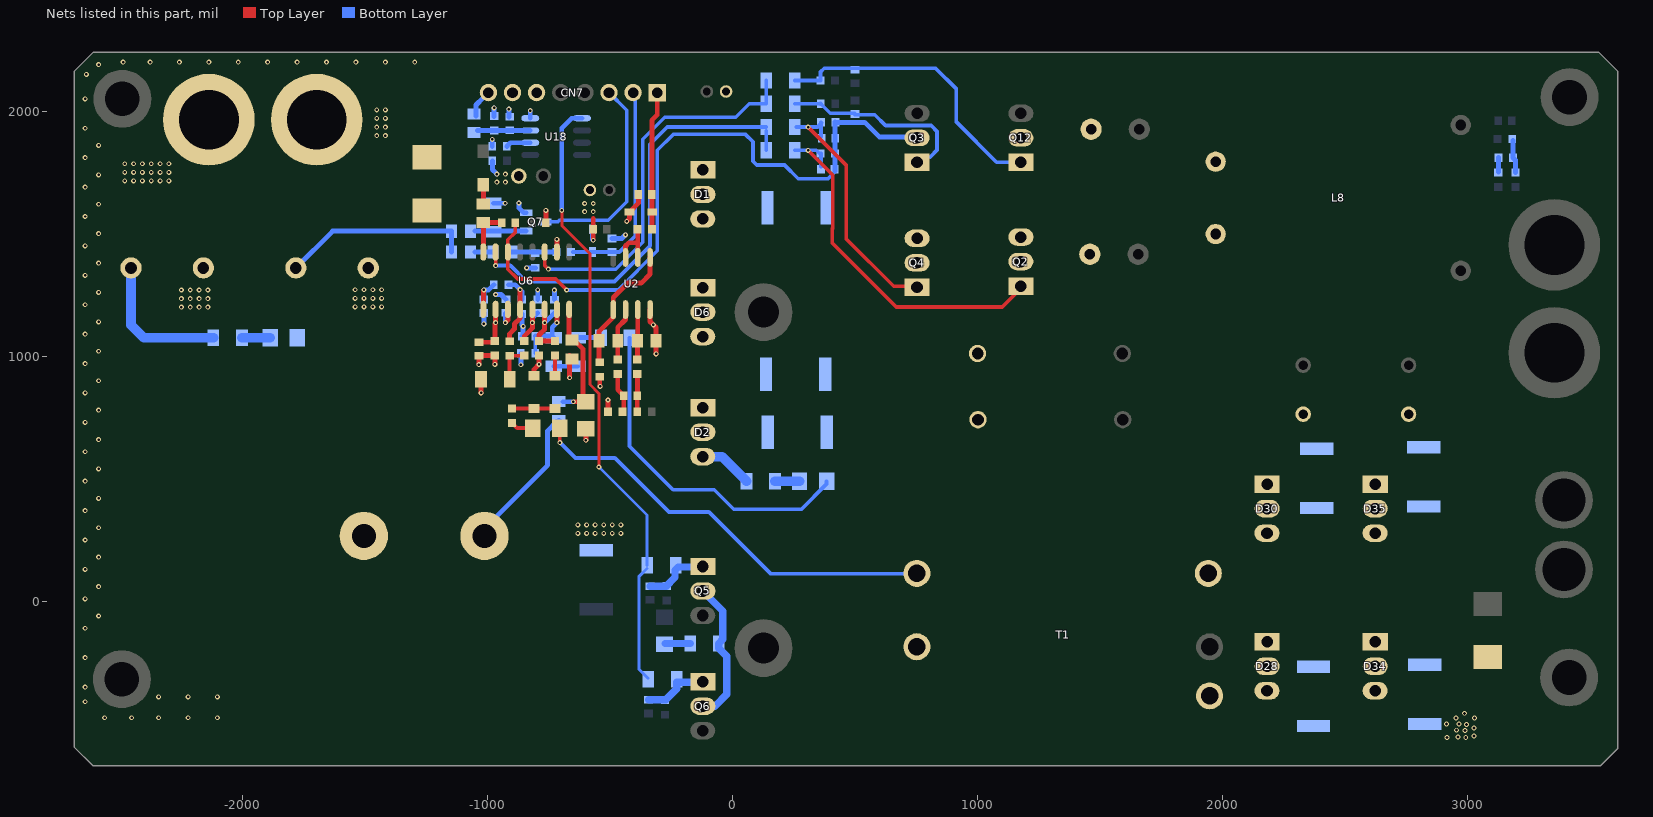
[diagram p0: the nets of this part, all layers, seen from the top]
# Altium PCB MISC89356.PcbDoc (part 2 of 3)
Units mil, origin at the board's own origin, x right, y up, seen from the top; angles counter-clockwise.
Board outline 6299.21 x 2912.91 mil, 4 copper layers (Top Layer, GND02, PWR03, Bottom Layer); 128 components, 68 nets, 313 pads, 200 vias.

## Via types
v1: diameter 20, hole 10, Top Layer to Bottom Layer, tented both sides, 177 vias
v2: diameter 20, hole 12, Top Layer to Bottom Layer, 13 vias
v3: diameter 20, hole 10, Top Layer to Bottom Layer, 10 vias

## Nets (pads, with @x,y where several pads share a name; then routed paths per layer and width w, separated by ;. In a path a pad name is that pad's centre, name@x,y a point inside that pad or via, vN(x,y) a via of type N, cw(c..) or ccw(c..) an arc to the next point about the centre after c; other vN are vias at no path point) (continued)
GND: C3.2 C5.2 C10.1 C11.2 C13.1 C14.1 C17.1 C18.1 C19.2 C20.2 C21.1 C27.1 C43.1 C44.2 C72.1 C74.2 C75.2 C169.2 CN7.6 D4.2 D12.2 D15.2 J6.2 Q7.2 R1.1 R4.1 R5.1 R7.2 R12.1 R15.2 R28.2 R29.2 R30.1 R34.2 R145.2 R186.2 R237.1 R271.1 R295.2 U2.4 U6.10 U18.4 | length 1778.5
  Top Layer w20: v1(-1035.15,968) C10.1@-1035.15,1003.69 -1034.46,1004.38 R1.1@-970.15,1004.38 v1(-970.15,968.69) ; v1(-1026.58,852.56) R15.2@-1026.58,908.69 ; D4.2@-810.15,921.96 -810.15,948.69 v1(-790.15,968.69) R12.1@-790.15,1004.38 ; C17.1@-762.04,1547 v1(-762.04,1596.89) ; U6.10@-717.15,1427 v1(-717.15,1478.69) ; v1(-665.15,914) R5.1@-665.15,1004.38 ; v3(-599.15,659.15) C27.1@-599.15,705.88 ; v1(-568.82,1475.11) C20.2@-568.82,1520 -568.82,1564.89 ; R34.2@-542.15,923.69 -542.15,880.09 v1(-541,879) v1(-541,879) ; R186.2@-508.59,776.01 v1(-508.59,823.32) ; v1(-432.15,1552) -421.04,1563.11 D12.2@-421.04,1590 -384.7,1626.34 C43.1@-384.7,1662 ; U2.4@-337.15,1192 -337.15,1143.44 v1(-323.71,1130) -312.63,1118.92 R145.2@-312.63,1065 v1(-312.63,1011.08)
  Bottom Layer w20: v1(-1015.15,1133.69) C13.1@-1015.15,1178.58 ; R237.1@-980.8,1858 v3(-980.8,1886.8) ; R271.1@-980.51,1799 -980.51,1763.51 v1@-963,1746 ; R28.2@-976.36,1626.05 v3(-928.05,1626.05) ; R295.2@-973.15,1979.66 v3(-973.15,2014.85) ; v1(-967.15,1253.69) -945.04,1253.69 C19.2@-925.15,1233.8 ; C21.1@-913.15,1977.56 v3(-913.15,2010.15) ; v1(-872.15,1627) -872.15,1607 -852.26,1587.11 Q7.2@-842.15,1587.11 ; C3.2@-870.49,1746 C3.2@-869,1746 ; v1(-864.35,967) R4.1@-864.35,1013.8 ; C11.2@-860.15,1083.69 -855.15,1088.69 v1(-855.15,1123.69) -860.15,1128.69 R7.2@-860.15,1174.38 ; v3(-840.61,1362.61) R29.2@-804.85,1362.61 ; U18.4@-825.76,1973 v3(-825.76,2004.24) ; C14.1@-795.15,1233.69 v1(-795.15,1272.58) ; C18.1@-727.15,1232.8 v1(-727.15,1271.69) ; D15.2@-572.15,1519.44 -572.15,1478.44 v1(-568.82,1475.11) ; C72.1@-492.15,1482.22 -451.93,1482.22 v1(-437.15,1497)
  other v1: -2562.15,-473 -2452.15,-473 -2342.15,-473 -2222.15,-473 -2102.15,-473 -2642.15,-408 -2342.15,-388 -2222.15,-388 -2102.15,-388 -2642.15,-348 -2642.15,-228 -2642.15,-108 -2587.15,-58 -2642.15,12 -2587.15,62 -2642.15,132 -2587.15,182 -2642.15,252 -631.15,279 -596.15,279 -561.15,279 -526.15,279 -491.15,279 -456.15,279 -2587.15,302 -631.15,314 -596.15,314 -561.15,314 -526.15,314 -491.15,314 -456.15,314 -2642.15,372 -2587.15,422 -2642.15,492 -2587.15,542 -2642.15,612 -2587.15,662 -2642.15,732 -2587.15,782 -2642.15,852 -2587.15,902 -2642.15,972 -2587.15,1022 -2642.15,1092 -2587.15,1142 -2249.15,1202 -2213.15,1202 -2177.15,1202 -2141.15,1202 -1540.15,1203 -1504.15,1203 -1468.15,1203 -1432.15,1203 -2642.15,1212 -2249.15,1237 -2213.15,1237 -2177.15,1237 -2141.15,1237 -1540.15,1238 -1504.15,1238 -1468.15,1238 -1432.15,1238 -2587.15,1262 -2249.15,1272 -2213.15,1272 -2177.15,1272 -2141.15,1272 -1540.15,1273 -1504.15,1273 -1468.15,1273 -1432.15,1273 -2642.15,1332 -2587.15,1382 -2642.15,1452 -2587.15,1502 -2642.15,1572 -603.71,1592 -568.71,1592 -2587.15,1622 -603.71,1625 -568.71,1625 -2642.15,1692 -962.15,1712 -927.15,1712 -2480.15,1717 -2444.15,1717 -2408.15,1717 -2372.15,1717 -2336.15,1717 -2300.15,1717 -2587.15,1742 -962.15,1745 -927.15,1745 -2480.15,1752 -2444.15,1752 -2408.15,1752 -2372.15,1752 -2336.15,1752 -2300.15,1752 -2480.15,1787 -2444.15,1787 -2408.15,1787 -2372.15,1787 -2336.15,1787 -2300.15,1787 -2642.15,1812 -2587.15,1862 -2642.15,1932 -2642.15,2052 -2637.15,2152 -2587.15,2192 -2487.15,2202 -2377.15,2202 -2257.15,2202 -2137.15,2202 -2017.15,2202 -1897.15,2202 -1777.15,2202 -1657.15,2202 -1537.15,2202 -1417.15,2202 -1297.15,2202
LLC_I: C6.1 C12.1 C15.1 T1.3 | length 1733.6
  Top Layer w15: v3(-704.91,649.09) C15.1@-704.91,708.69
  Bottom Layer w15: v3@-705,650 -704.5,649.5 -641.5,586.5 -480.5,586.5 -260,366 -97,366 154,115 746.98,115 T1.3@747.31,114.67
LO: R49.1 R73.1 U18.5 | length 2504.9
  Top Layer w12: v1@-697.15,1595 v1(-697.15,1597) ; v1@-697,1595 -697,1535 -582,1420 -582,886 -546,850 -546,554 v3@-547,553 ; v3@-547,550 v3(-546,550)
  Bottom Layer w12: v3(-546,550) v3@-545.15,550 ; v3@-545.57,550.43 v3@-545.15,550 ; R73.1@-349,136 -383,102 -383,-274 R49.1@-345,-312 ; R73.1@-349,148.51 -349,353.85 v3@-545.15,550
  Bottom Layer w20: v1(-697.15,1597) -697.15,1932.59 -656.74,1973 U18.5@-614.54,1973
NetC1_1: C1.1 C2.1 F1.1 R41.2 R42.2 R43.2 R44.2
  other v2: 2991,-554 2914,-553 2959,-551 3025,-548 2988,-526 2953,-524 3025,-515 2994,-500 2913,-499 2964,-499 3027,-475 2952,-474 2986,-455
NetC4_1: C4.1 R10.2 | length 101.6
  Bottom Layer w30: C4.1@-275.06,-170.15 R10.2@-173.44,-170.15
NetC5_1: C5.1 R11.2 | length 115
  Bottom Layer w40: R11.2@-2002.15,1077 C5.1@-1887.15,1077
NetC7_1: C7.1 R47.2 | length 100
  Bottom Layer w40: R47.2@172.85,492 C7.1@272.85,492
NetC7_2: C7.2 C8.1 C73.1 Q2.2 Q4.2 R17.1 R22.2 R45.2 R46.2 | length 1406.6
  Bottom Layer w15: R17.1@-420.71,1077 -420.71,634.71 -243,457 -75,457 4,378 281,378 383.09,480.09 C7.2@383.09,492
NetC9_1: C9.1 Q6.1 R49.2 R98.2 | length 251.6
  Bottom Layer w30: C9.1@-343,-400.3 -273.3,-400.3 -228,-355 -228,-329 -139,-329 Q6.1@-137,-327
NetC10_2: C10.2 R1.2 U6.2 | length 197.6
  Top Layer w20: C10.2@-1035.15,1058.8 -975.04,1058.8 R1.2@-970.15,1063.69 -970.15,1135.69 v1(-967.15,1138.69) U6.2@-967.15,1193
NetC11_1: C11.1 R4.2 R24.2 U6.7 | length 264.5
  Top Layer w20: v1(-717.15,1138.69) U6.7@-717.15,1193
  Bottom Layer w15: R4.2@-805.04,1013.8 C11.1@-805.04,1083.69
  Bottom Layer w20: C11.1@-805.04,1083.69 R24.2@-736.23,1083.69 ; R24.2@-730.15,1077.61 R24.2@-736.23,1083.69 ; v1(-717.15,1138.69) -736.23,1119.61 R24.2@-736.23,1083.69
NetC13_2: C13.2 R6.2 U6.1 | length 165.9
  Top Layer w20: U6.1@-1017.15,1193 v1@-1017.15,1270.58
  Bottom Layer w20: C13.2@-1015.15,1233.69 v1(-1015.15,1272.58) -995.57,1272.58 R6.2@-974.46,1293.69
NetC14_2: C14.2 R8.2 U6.5 | length 192
  Top Layer w20: R8.2@-850.15,1063.69 -850.15,1083.69 -817.15,1116.69 v1(-817.15,1138.69) U6.5@-817.15,1193
  Bottom Layer w20: v1(-817.15,1138.69) -817.15,1156.58 C14.2@-795.15,1178.58
NetC15_2: C15.2 R14.1 | length 93.6
  Top Layer w15: R14.1@-900.15,729.38 -879.46,708.69 C15.2@-815.15,708.69
NetC16_2: C16.2 R23.1 U6.16 | length 195
  Top Layer w20: U6.16@-1017.15,1427 R23.1@-1017.15,1547 C16.2@-942.15,1547
NetC18_2: C18.2 R12.2 R13.2 U6.6 | length 260
  Top Layer w20: U6.6@-767.15,1193 v1(-767.15,1138.69) -767.15,1111.69 -790.15,1088.69 R12.2@-790.15,1063.69 R13.2@-725.15,1063.69
  Bottom Layer w20: v1(-767.15,1138.69) -766.15,1138.69 C18.2@-727.15,1177.69
NetC19_1: C19.1 U6.3 | length 96.5
  Top Layer w20: v1(-927.15,1138.69) -917.15,1148.69 U6.3@-917.15,1193
  Bottom Layer w20: v1(-927.15,1138.69) C19.1@-927.15,1176.69
NetC21_2: C21.2 L12.2 R295.1 U18.3 | length 215.2
  Bottom Layer w20: L12.2@-1041,1923 U18.3@-825.76,1923
NetC22_1: C22.1 Q5.1 R73.2 R86.2 | length 228.6
  Bottom Layer w30: C22.1@-337.15,63.55 -271.45,63.55 -235,100 -235,129 -222,142 Q5.1@-158,142
NetC23_1: C23.1 Q2.1 R19.2 R25.1 | length 1600.9
  Top Layer w15: v1(307.85,1842) 407.85,1742 407.85,1523 ; 407,1523 407,1463 667,1203 820,1203 ; 725.85,1203 820,1203 ; Q2.1@1185.46,1288 1100.46,1203 820,1203
  Bottom Layer w15: R19.2@252.85,1842 v1(307.85,1842) 341,1842 R25.1@357,1826 ; C23.1@360.45,1774.85 R25.1@360.45,1829
NetC24_1: C24.1 Q4.1 R20.2 R325.1 | length 1058
  Top Layer w15: v1(307.85,1937) 462.85,1782 462.85,1481.15 657,1287 Q4.1@752,1287
  Bottom Layer w15: R20.2@259.92,1937 v1(307.85,1937) 346,1937 R325.1@360.23,1951.23 ; C24.1@360.23,1897.77 R325.1@360.23,1951.23 ; R325.1@360.23,1956 R325.1@360.23,1951.23 ; R325.1@363,1954 R325.1@360.23,1951.23
NetC25_1: C25.1 Q3.1 R32.1 R33.2 | length 765.7
  Bottom Layer w15: R33.2@252.85,2032 R32.1@358.54,2032 ; R32.1@359.23,2032 398.23,1993 496,1993 C25.1@497,1992 ; C25.1@499.15,1987 580,1987 624.07,1942.93 810.07,1942.93 834,1919 834,1843 806,1815 ; Q3.1@756.85,1788 757.85,1787 Q3.1@782.85,1787
  Bottom Layer w20: R32.1@358.54,2032 R32.1@359.23,2032
NetC26_1: C26.1 Q12.1 R21.2 R302.1 | length 1211.7
  Bottom Layer w15: R21.2@252.85,2127 R302.1@358.54,2127 358.54,2162 373.54,2177 827.85,2177 912.85,2092 912.85,1957.15 1077,1793 Q12.1@1185.32,1793
NetC27_2: C27.2 R2.1 R5.2 U6.8 | length 494.8
  Top Layer w20: U6.8@-667.15,1193 -667.15,1065.69 R5.2@-665.15,1063.69 ; R5.2@-655.15,1067.41 -646.41,1067.41 -610,1031 -610,821 C27.2@-609,820 ; v3(-649.88,816.12) C27.2@-599.15,816.12
  Bottom Layer w20: R2.1@-692.12,816.12 v3(-649.88,816.12)
NetC78_1: C78.1 R27.2 R186.1 | length 146.1
  Top Layer w20: -468.71,910 -468.71,865.33 C78.1@-444.39,841.01 -444.39,780.9 R186.1@-449.28,776.01
NetC78_2: C78.2 R3.2 R338.1 | length 134.2
  Top Layer w20: R338.1@-389.28,776.01 C78.2@-389.28,841.01 -388.71,841.57 -388.71,910
NetD1_1: D1.1 D1.3 D2.1 D2.3 D6.1 D6.3 L4.2 Q5.2 Q6.2 R10.1 R47.1 | length 785.2
  Bottom Layer w30: Q6.2@-121.62,-426 -72.07,-426 -23.59,-377.52 -23.59,-222.71 -57,-189.3 R10.1@-57,-170.15 -40,-153.15 -40,-37.62 Q5.2@-121.62,44
  Bottom Layer w40: D2.3@-93,592 -43.58,592 R47.1@56.42,492
NetD1_2: D1.2 R45.1
NetD2_2: D2.2 R46.1
NetD3_1: D3.1 R13.1 | length 82.4
  Top Layer w15: D3.1@-725.15,921.96 R13.1@-725.15,1004.38
NetD3_2: D3.2 D4.1 R14.2 | length 175
  Top Layer w15: R14.2@-900.15,788.69 D4.1@-810.15,788.69 D3.2@-725.15,788.69
NetD5_1: D5.1 R23.2 | length 78.9
  Top Layer w20: R23.2@-1017.15,1623.08 D5.1@-1017.15,1702
NetD6_2: D6.2 R22.1
NetD28_1: D28.1 D28.3 D34.1 D34.3 T1.8
NetD28_2: D28.2 R42.1
NetD30_1: D30.1 D30.3 D35.1 D35.3 T1.10
NetD30_2: D30.2 R44.1
NetD34_2: D34.2 R41.1
NetD35_2: D35.2 R43.1
NetL8_4: L8.4 T1.4
NetQ7_1: Q7.1 R18.1 R28.1 | length 209.8
  Bottom Layer w20: R18.1@-1051.95,1512.31 -927.15,1512.31 Q7.1@-842.15,1512.31
NetR3_1: R3.1 R145.1 U2.3 | length 204.4
  Top Layer w20: R3.1@-388.71,986.08 R145.1@-388.71,1065 ; R145.1@-387.15,1066.57 U2.3@-387.15,1192
NetR6_1: R6.1 R7.1 R9.1 U6.4 | length 327.3
  Top Layer w20: R9.1@-910.15,1063.35 -910.15,1093.69 -890.15,1113.69 -890.15,1133.69 -867.15,1156.69 U6.4@-867.15,1193 v1(-867.15,1273.69)
  Bottom Layer w20: R6.1@-915.15,1293.69 -887.15,1293.69 v1(-867.15,1273.69) -860.15,1266.69 R7.1@-860.15,1233.69
NetR8_1: R8.1 R9.2 R15.1 | length 155.5
  Top Layer w15: R15.1@-910.15,908.69 R9.2@-910.15,1004.04 -850.49,1004.04 R8.1@-850.15,1004.38
NetR16_1: R16.1 R17.2 | length 94.4
  Bottom Layer w20: R16.1@-632.15,1077.61 R17.2@-537.75,1077.61
NetR16_2: R16.2 R24.1 | length 98
  Bottom Layer w20: R24.1@-730.15,961.17 R16.2@-632.15,961.17
NetR26_1: R26.1 R35.2 | length 73.9
  Bottom Layer w20: R26.1@-1051.06,1427.11 R35.2@-977.15,1427.11
NetR27_1: R27.1 R142.2 U2.2 | length 219
  Top Layer w20: R27.1@-468.71,986.08 R142.2@-468.71,1065 -468.71,1120 -437.15,1151.57 U2.2@-437.15,1192
NetR29_1: R29.1 R35.1 R39.1 | length 173.9
  Bottom Layer w20: R35.1@-901.06,1427.11 -807.15,1427.11 R39.1@-727.15,1427.11
NetR34_1: R34.1 R142.1 U2.1 U2.5 | length 543.6
  Top Layer w20: R34.1@-544.8,979.65 R142.1@-544.8,1065 -544.8,1103.92 -487.15,1161.57 U2.1@-487.15,1192 -487.15,1241.57 -428.71,1300 -373.71,1300 -337.15,1336.57 U2.5@-337.15,1405
NetR40_2: R40.2 R53.2 R106.1 | length 134.1
  Bottom Layer w20: R40.2@3183.85,1882 R106.1@3183.85,1812 3193.85,1802 R53.2@3193.85,1752
NetR106_2: R106.2 R148.1 | length 59.3
  Bottom Layer w20: R148.1@3124.54,1752.69 R106.2@3124.54,1812
NetR147_1: R147.1 U2.6 U2.7 | length 215.6
  Top Layer w20: U2.7@-437.15,1405 -437.15,1451.57 -423.71,1465 -387.15,1465 ; U2.6@-387.15,1405 -387.15,1465 ; R147.1@-387.15,1518.44 -387.15,1465
NetR237_2: R237.2 U18.2 | length 101.9
  Bottom Layer w20: R237.2@-921.49,1858 -906.49,1873 U18.2@-825.76,1873
PV+: F6.1 J6.1
  other v1: -1452.15,1902 -1417.15,1902 -1452.15,1937 -1417.15,1937 -1452.15,1972 -1417.15,1972 -1452.15,2007 -1417.15,2007
PV-I: C43.2 CN7.1 D12.1 R147.2 | length 566.4
  Top Layer w20: R147.2@-329.4,1520 -329.4,1590 -329.4,1662 -329.4,1964.75 -307.66,1986.49 -307.66,2010 CN7.1@-307.66,2077.44
PV-INT: CN7.3 Q7.3 | length 840.8
  Bottom Layer w15: Q7.3@-763.41,1549.71 -763.12,1550 -714,1550 -707,1557 -507.15,1557 -432.15,1632 -432.15,2005.08 CN7.3@-504.5,2077.44
PV-OVP: C75.1 C169.1 F6.2 L4.1 R2.2 R11.1 R18.2 R26.2 | length 1913.6
  Bottom Layer w20: C75.1@-1782.15,1362 -1632.04,1512.11 -1146.52,1512.11 R18.2@-1146.52,1512 R26.2@-1146.52,1427 ; L4.1@-993,319 -755,557 -755,698 R2.2@-717,736 ; R2.2@-715.39,734.39 R2.2@-709,740.77
  Bottom Layer w40: C169.1@-2454.81,1362.01 -2454.81,1129.66 -2402.15,1077 R11.1@-2118.58,1077
PV-U: C72.2 CN7.2 D15.1 R39.2 | length 869.9
  Bottom Layer w12: CN7.2@-406.08,2077.44 CN7.2@-397.15,2068.5
  Bottom Layer w15: R39.2@-651.06,1427.11 D15.1@-572.15,1427.11 C72.2@-492.15,1427.11 -462.15,1427.11 -397.15,1492.11 CN7.2@-397.15,2068.5
PWM-H: CN7.7
PWM-L: CN7.8 L12.1 | length 116.7
  Bottom Layer w15: CN7.8@-1016.94,2057.13 CN7.8@-996.63,2077.44
  Bottom Layer w20: L12.1@-1047.15,1981.66 -1047.15,2026.92 CN7.8@-1016.94,2057.13
Q4G: R19.1 R20.1 U6.15 | length 1769.7
  Top Layer w15: v1(-967.15,1371.69) U6.15@-967.15,1427
  Bottom Layer w15: v1(-967.15,1371.69) -906.84,1371.69 -842.15,1307 -482.15,1307 -337.15,1452 -337.15,1867 -267.15,1937 R20.1@136.42,1937 ; R19.1@136.42,1842 R20.1@136.42,1922
Q12G: R21.1 R33.1 U6.11 | length 1585.4
  Top Layer w15: U6.11@-767.15,1427 -767.15,1372 v1(-752.15,1357)
  Bottom Layer w15: v1(-752.15,1357) -477.15,1357 -367.15,1467 -367.15,1887 -277.15,1977 12.85,1977 67.85,2032 R33.1@136.42,2032 R21.1@136.42,2127
T1H: C16.1 C23.2 C24.2 L8.3 Q2.3 Q3.2 Q4.3 Q12.2 R25.2 R325.2 U6.14 | length 2772.2
  Top Layer w15: C16.1@-887.04,1547 -887.04,1507.11 -917.15,1477 U6.14@-917.15,1427 -917.15,1357 -877.15,1317 -722.15,1317 v1(-677.15,1272)
  Bottom Layer w15: v1(-677.15,1272) -467.15,1272 -307.15,1432 -307.15,1842 -242.15,1907 52.85,1907 82.85,1877 82.85,1797 97.85,1782 212,1782 268,1726 389,1726 419,1756 C23.2@419,1764.85
  Bottom Layer w20: C23.2@417.85,1757.85 R25.2@417.85,1829 417.85,1842 417.85,1956.85 R325.2@418,1957 ; R325.2@419.54,1956 539,1956 598,1897 Q3.2@748,1897
pads on no net: L8.8 L8.11 U6.9 U6.13 U18.6 U18.7 U18.8

## Polygon pours and split planes (outlines as drawn)
NetC1_1 on Top Layer "BottomLayer-No Net" (solid, remove dead copper): 2042,-93 2042,-520 2069,-547 2096,-574 2134,-574 3051,-574 3111,-514 3176,-449 3176,-333 3176,-203 3157,-184 3145,-172 3110,-172 2976,-172 2891,-87 2852,-48 2852,176 2852,832 2806,878 2802,882 2790,882 2150,882 2098,830 2042,774 2042,-93
B+ on Top Layer "BottomLayer-No Net" (solid, remove dead copper): 2973,205 2973,-18 3000,-45 3018,-63 3035,-63 3477,-63 3502,-38 3520,-20 3520,70 3520,210 3497,233 3477,253 3417,253 3301,253 3255,299 3238,316 3238,646 3238,712 3263,737 3283,757 3353,757 3457,757 3523,823 3555,855 3555,969 3555,1123 3512,1166 3475,1203 3388,1203 3129,1203 3072,1146 2973,1047 2973,205
PV-OVP on Top Layer "BottomLayer-No Net" (solid, remove dead copper): -2552,1456 -2552,619 -2468,535 -2430,497 -2351,497 -1401,497 -1282,378 -1255,351 -1255,265 -1255,164 -1203,112 -1175,84 -1081,84 -901,84 -867,118 -851,134 -851,177 -851,552 -1118,819 -1130,831 -1130,888 -1130,1622 -1144,1636 -1153,1645 -1184,1645 -2457,1645 -2526,1576 -2552,1550 -2552,1456
NetD1_1 on Top Layer "BottomLayer-No Net" (solid, remove dead copper): -2037,172 -2037,96 -2037,-418 -1970,-485 -1869,-586 -296,-586 170,-586 240,-516 334,-422 334,-175 334,1721 216,1839 182,1873 53,1873 -137,1873 -197,1813 -208,1802 -208,1753 -208,590 -268,530 -311,487 -512,487 -688,487 -713,462 -742,433 -742,399 -742,89 -847,-16 -869,-38 -1063,-38 -1297,-38 -1367,32 -1378,43 -1378,220 -1378,352 -1422,396 -1436,410 -1486,410 -1894,410 -1992,312 -2038,266 -2038,175
NetL8_4 on Top Layer "BottomLayer-No Net" (solid, remove dead copper, pour order 1000): 425,703 425,-196 476,-247 507,-278 557,-278 816,-278 831,-263 840,-254 840,-216 840,-80 812,-52 800,-40 746,-40 689,-40 656,-7 638,11 638,35 638,583 689,634 706,651 803,651 1742,651 1899,808 1934,843 1934,966 1934,1134 2013,1213 2077,1277 2077,1426 2077,1571 2046,1602 2041,1607 1960,1607 1813,1607 1772,1566 1741,1535 1741,1425 1741,1344 1596,1199 1520,1123 1132,1123 666,1123 456,913 425,882 425,703
PV+ on Top Layer "Bottom Layer-No Net 2" (hatched 90Degree grid 8 track 10, remove dead copper, pour order 1026): -1882.15,2172 -1901.15,2153 -1901.15,1748 -1880.15,1727 -1157.15,1727 -1142.15,1742 -1142.15,2162 -1152.15,2172
GND on Top Layer "Bottom Layer-No Net 2" (solid, remove dead copper, pour order 1025): -629.71,1750 -644.71,1735 -644.71,1450 -634.71,1440 -559.71,1440 -554.71,1445 -554.71,1740 -564.71,1750
+12V on Top Layer "Bottom Layer-No Net 2" (solid, remove dead copper, pour order 1024): -528.71,1780 -458.71,1780 -448.71,1770 -448.71,1635 -468.71,1615 -468.71,1360 -473.71,1355 -518.71,1355 -528.71,1365 -528.71,1715 -538.71,1725 -538.71,1770
GND on Top Layer "BOTTOM-No Net" (solid, remove dead copper, pour order 1064): -2592.15,1692 -2657.15,1757 -2657.15,2177 -2627.15,2207 -1957.15,2207 -1942.15,2192 -1942.15,1707 -1957.15,1692
+12V on Top Layer "Bottom Layer-No Net 2" (solid, remove dead copper, pour order 1000): -448.71,1770 -448.71,1963.57 -472.15,1987 -627.15,1987 -667.15,2027 -667.15,2107 -682.15,2122 -727.15,2122 -742.15,2107 -742.15,2017 -827.15,1932 -827.15,1572 -812.15,1557 -807.15,1557 -807.15,1562 -797.15,1572 -797.15,1592 -707.15,1682 -707.15,1762 -687.15,1782 -550.71,1782 -525.71,1757 -452.15,1757
T1H on Top Layer "BottomLayer-No Net" (solid, remove dead copper, pour order 1001): 527,1989 527,1976 527,1535 584,1478 622,1440 841,1440 1312,1440 1350,1478 1570,1698 1930,1698 2001,1698 2034,1731 2059,1756 2059,1822 2059,2132 2038,2153 2006,2185 1949,2185 610,2185 543,2118 527,2102 527,1989
BAT- on GND02 "BottomLayer-No Net" (solid, remove dead copper, pour order 1005): 591,788 591,584 578,571 675,668 764,668 1813,668 1875,606 1906,637 1922,637 1922,753 1928,759 1727,960 1643,960 709,960 638,889 590,841 590,793